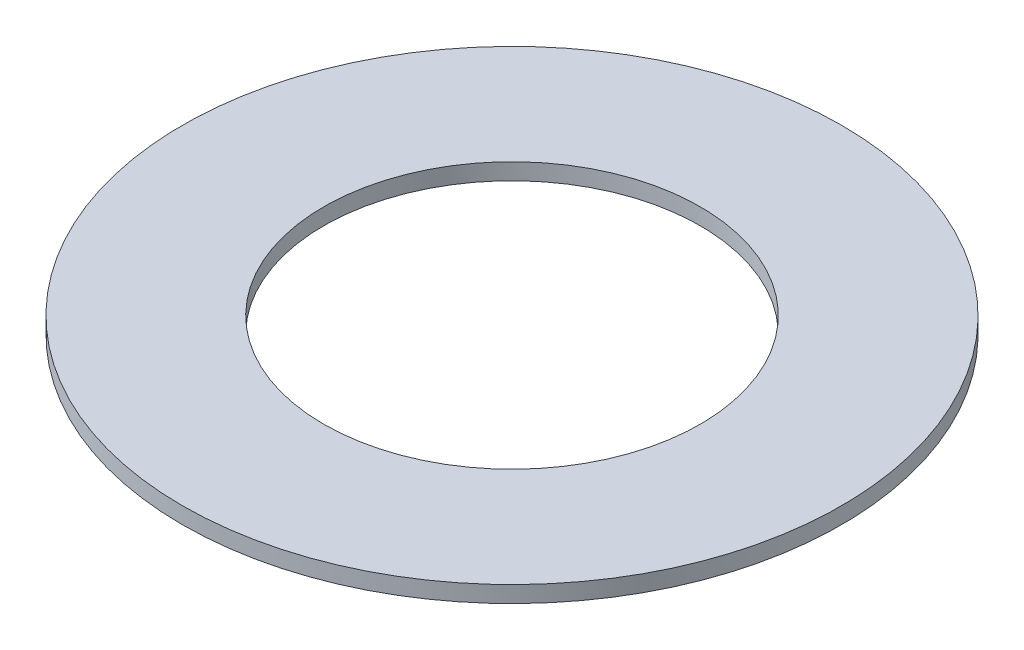
from build123d import *

# Parameters (mm, degrees)
SKETCH1_R           = 7
SKETCH1_R_2         = 4
BOSS_EXTRUDE1_DEPTH = 0.35


with BuildPart() as part:
    # Sketch1 → Boss-Extrude1 (new body)
    with BuildSketch(Plane(origin=(0, 0, 0), x_dir=(1, 0, 0), z_dir=(0, 1, 0))):
        with Locations(Location((0, 0, 0), (0, 0, 270))):
            Circle(SKETCH1_R)
        with Locations(Location((0, 0, 0), (0, 0, 270))):
            Circle(SKETCH1_R_2, mode=Mode.SUBTRACT)
    extrude(amount=BOSS_EXTRUDE1_DEPTH)


solid = part.part
